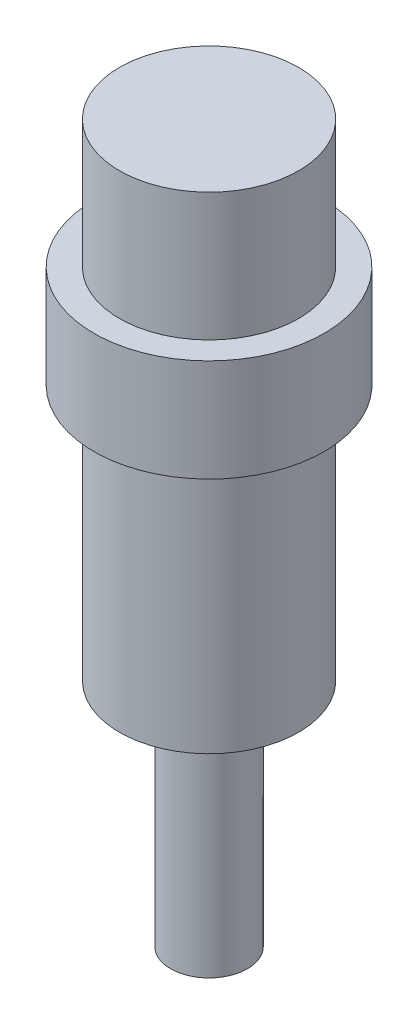
from build123d import *


with BuildPart() as part:
    # 草图3 → 旋转19 (revolve)
    with BuildSketch(Plane.XY, mode=Mode.PRIVATE) as revolve_19_sk:
        Polygon((0, 10.070696149), (3.5, 10.070696149), (3.5, 5.070696149), (4.5, 5.070696149), (4.5, 1.070696149), (3.5, 1.070696149), (3.5, -8.929303851), (1.5, -8.929303851), (1.5, -17.929303851), (0, -17.929303851), align=None)
    revolve(revolve_19_sk.sketch.rotate(Axis((0, 0, 0), (0, 1, 0)), 90), axis=Axis((0, 0, 0), (0, 1, 0)))


solid = part.part
